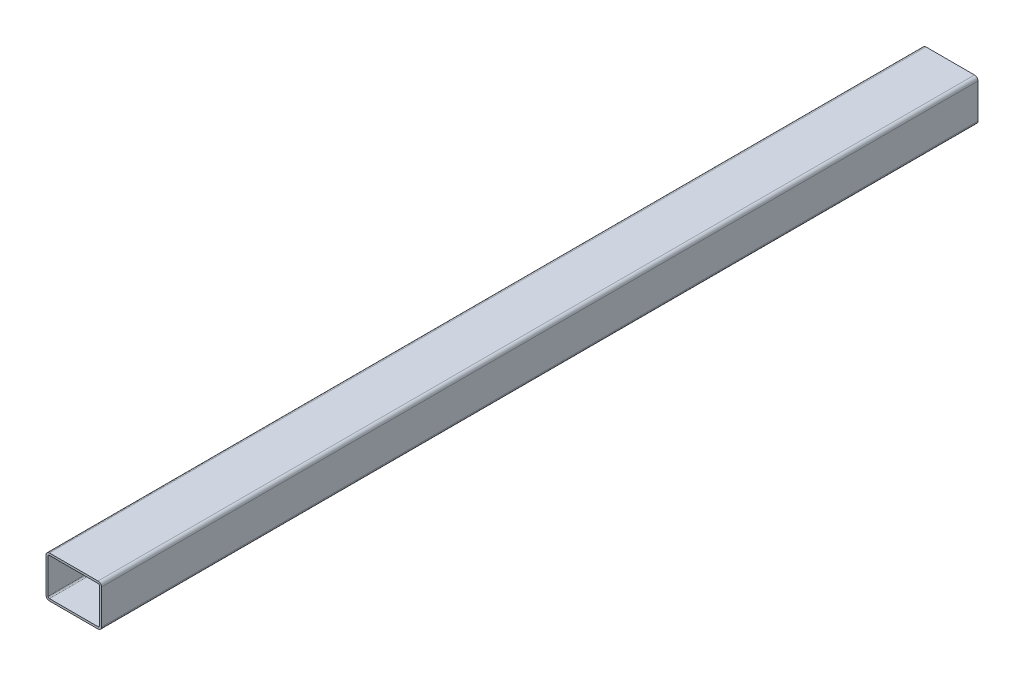
SolidWorks part; units mm, degrees
material "1023 碳钢板 (SS)"
ref_plane "前视基准面" through (0, 0, 0) normal (0, 0, 1) x (1, 0, 0)
ref_plane "上视基准面" through (0, 0, 0) normal (0, 1, 0) x (1, 0, 0)
ref_plane "右视基准面" through (0, 0, 0) normal (1, 0, 0) x (0, 0, -1)
sketch "草图1" plane through (0, 0, 0) normal (0, 0, 1) x (1, 0, 0)
  line L1 (40, 30) -> (-40, 30)
  line L2 (40, 30) -> (40, -30)
  line L3 (40, -30) -> (-40, -30)
  line L4 (-40, 30) -> (-40, -30)
  line L5 (40, 30) -> (-40, -30) construction
  line L6 (40, -30) -> (-40, 30) construction
  point P0 (0, 0)
  dimension "D1" = 80
  dimension "D2" = 60
extrude "凸台-拉伸1" add sketch "草图1" along normal blind 1264
fillet "圆角1" radius 5 4 edges at (40, -30, 632) (-40, -30, 632) (-40, 30, 632) (40, 30, 632)
shell "抽壳1" thickness 3
